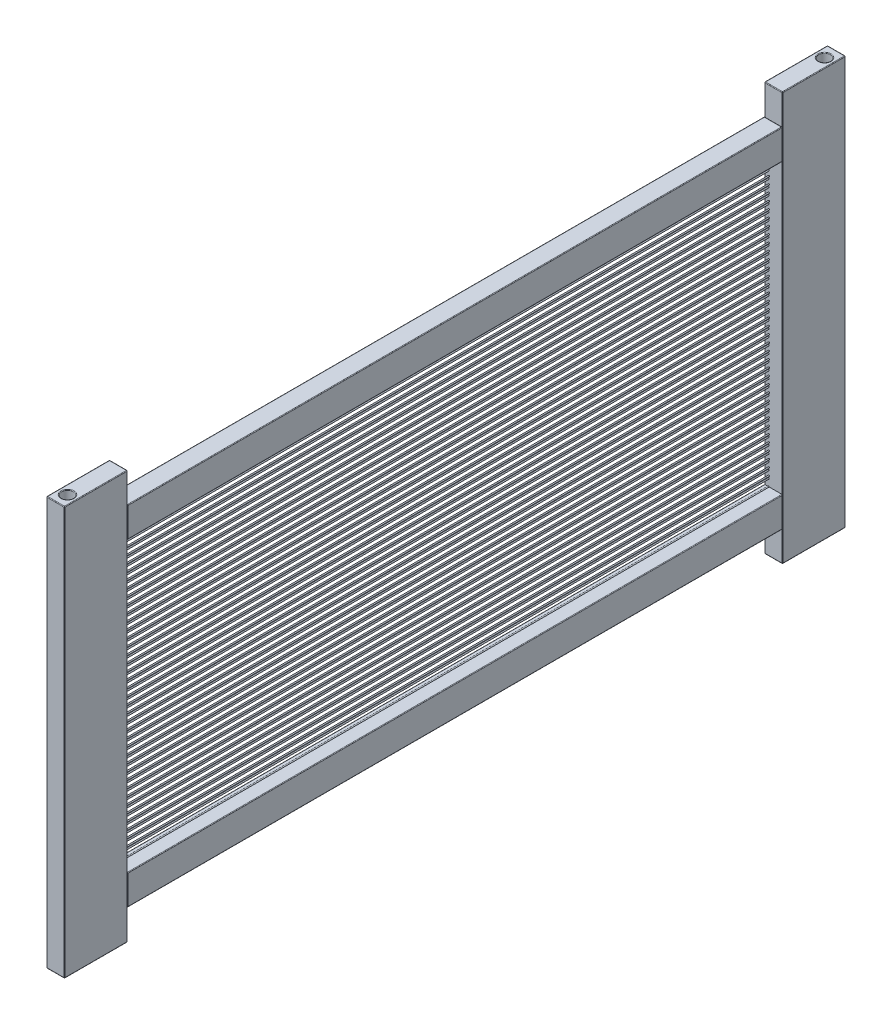
from build123d import *

# Parameters (mm, degrees)
SKETCH_1_W          = 30
SKETCH_1_H          = 105
EXTRUDE_1_DEPTH     = 680
EXTRUDE_1_2_DEPTH   = 680
SKETCH_2_R          = 10
CUT_EXTRUDE_1_DEPTH = 1421.873410969
SKETCH_6_W          = 30
SKETCH_6_H          = 50
EXTRUDE_2_DEPTH     = 1090
EXTRUDE_2_2_DEPTH   = 1090
SKETCH_7_R          = 1
EXTRUDE_3_DEPTH     = 1090
FILLET_1_R          = 1
FILLET_2_R          = 1
FILLET_3_R          = 1
FILLET_4_R          = 1


with BuildPart() as part:
    # 草图1 → 凸台-拉伸1 (new body)
    with BuildSketch(Plane(origin=(0, 0, 0), x_dir=(1, 0, 0), z_dir=(0, 1, 0))):
        Rectangle(SKETCH_1_W, SKETCH_1_H)
    extrude(amount=EXTRUDE_1_DEPTH)


with BuildPart() as body_2:
    # 草图1 → Extrude 1 2 (new body)
    with BuildSketch(Plane(origin=(0, 0, 0), x_dir=(1, 0, 0), z_dir=(0, 1, 0))):
        with Locations((0, 1195)):
            Rectangle(SKETCH_1_W, SKETCH_1_H)
    extrude(amount=EXTRUDE_1_2_DEPTH)


with BuildPart() as cut_extrude_1_tool:
    # 草图2 → 切除-拉伸1 (new, through all)
    with BuildSketch(Plane.XZ):
        with Locations(Location((0, 32.5, 0), (0, 0, 270))):
            Circle(SKETCH_2_R)
        with Locations(Location((0, -1227.5, 0), (0, 0, 270))):
            Circle(SKETCH_2_R)
    extrude(amount=-CUT_EXTRUDE_1_DEPTH)


with BuildPart() as part_1:
    add(part.part)

    # 切除-拉伸1: cut by cut_extrude_1_tool
    add(cut_extrude_1_tool.part, mode=Mode.SUBTRACT)

    # 圆角1
    fillet_1_edges = [part_1.edges().sort_by_distance(p)[0] for p in [
        (-15, 680, 0),
        (0, 680, 52.5),
        (0, 680, 42.5),
        (0, 0, 42.5),
        (15, 680, 0),
        (0, 0, 52.5),
        (-15, 0, 0),
        (0, 0, -52.5),
        (15, 0, 0),
        (0, 680, -52.5),
        (15, 340, 52.5),
        (-15, 340, 52.5),
        (-15, 340, -52.5),
        (15, 340, -52.5),
    ]]
    fillet(fillet_1_edges, radius=FILLET_1_R)


with BuildPart() as body_2_1:
    add(body_2.part)

    # 切除-拉伸1: cut by cut_extrude_1_tool
    add(cut_extrude_1_tool.part, mode=Mode.SUBTRACT)

    # 圆角3
    fillet_3_edges = [body_2_1.edges().sort_by_distance(p)[0] for p in [
        (-15, 680, -1195),
        (0, 680, -1142.5),
        (0, 680, -1217.5),
        (15, 680, -1195),
        (0, 0, -1142.5),
        (-15, 0, -1195),
        (0, 0, -1247.5),
        (15, 0, -1195),
        (0, 680, -1247.5),
        (15, 340, -1142.5),
        (-15, 340, -1142.5),
        (-15, 340, -1247.5),
        (15, 340, -1247.5),
    ]]
    fillet(fillet_3_edges, radius=FILLET_3_R)


with BuildPart() as body_3:
    # 草图6 → 凸台-拉伸2 (new body)
    with BuildSketch(Plane.XY.offset(-1142.5)):
        with Locations((0, 75)):
            Rectangle(SKETCH_6_W, SKETCH_6_H)
    extrude(amount=EXTRUDE_2_DEPTH)

    # 圆角4
    fillet_4_edges = [body_3.edges().sort_by_distance(p)[0] for p in [
        (0, 50, -1142.5),
        (15, 50, -597.5),
        (15, 75, -1142.5),
        (15, 100, -597.5),
        (-15, 75, -52.5),
        (0, 50, -52.5),
        (15, 75, -52.5),
        (-15, 100, -597.5),
        (-15, 75, -1142.5),
        (-15, 50, -597.5),
    ]]
    fillet(fillet_4_edges, radius=FILLET_4_R)


with BuildPart() as body_4:
    # 草图6 → Extrude 2 2 (new body)
    with BuildSketch(Plane.XY.offset(-1142.5)):
        with Locations((0, 605)):
            Rectangle(SKETCH_6_W, SKETCH_6_H)
    extrude(amount=EXTRUDE_2_2_DEPTH)

    # 圆角2
    fillet_2_edges = [body_4.edges().sort_by_distance(p)[0] for p in [
        (15, 580, -597.5),
        (15, 605, -1142.5),
        (15, 630, -597.5),
        (0, 630, -1142.5),
        (0, 630, -52.5),
        (-15, 605, -52.5),
        (15, 605, -52.5),
        (-15, 630, -597.5),
        (-15, 605, -1142.5),
        (-15, 580, -597.5),
    ]]
    fillet(fillet_2_edges, radius=FILLET_2_R)


with BuildPart() as body_5:
    # 草图7 → 凸台-拉伸3 (new body)
    with BuildSketch(Plane.XY.offset(-1142.5)):
        with Locations((-8, 568)):
            Circle(SKETCH_7_R)
        with Locations((-7.551054028, 583.993700245)):
            Circle(SKETCH_7_R)
        with Locations((-8, 556)):
            Circle(SKETCH_7_R)
        with Locations((-7.551054028, 571.993700245)):
            Circle(SKETCH_7_R)
        with Locations((-8, 544)):
            Circle(SKETCH_7_R)
        with Locations((-7.551054028, 559.993700245)):
            Circle(SKETCH_7_R)
        with Locations((-8, 532)):
            Circle(SKETCH_7_R)
        with Locations((-7.551054028, 547.993700245)):
            Circle(SKETCH_7_R)
        with Locations((-8, 520)):
            Circle(SKETCH_7_R)
        with Locations((-7.551054028, 535.993700245)):
            Circle(SKETCH_7_R)
        with Locations((-8, 508)):
            Circle(SKETCH_7_R)
        with Locations((-7.551054028, 523.993700245)):
            Circle(SKETCH_7_R)
        with Locations((-8, 496)):
            Circle(SKETCH_7_R)
        with Locations((-7.551054028, 511.993700245)):
            Circle(SKETCH_7_R)
        with Locations((-8, 484)):
            Circle(SKETCH_7_R)
        with Locations((-7.551054028, 499.993700245)):
            Circle(SKETCH_7_R)
        with Locations((-8, 472)):
            Circle(SKETCH_7_R)
        with Locations((-7.551054028, 487.993700245)):
            Circle(SKETCH_7_R)
        with Locations((-8, 460)):
            Circle(SKETCH_7_R)
        with Locations((-7.551054028, 475.993700245)):
            Circle(SKETCH_7_R)
        with Locations((-8, 448)):
            Circle(SKETCH_7_R)
        with Locations((-7.551054028, 463.993700245)):
            Circle(SKETCH_7_R)
        with Locations((-8, 436)):
            Circle(SKETCH_7_R)
        with Locations((-7.551054028, 451.993700245)):
            Circle(SKETCH_7_R)
        with Locations((-8, 424)):
            Circle(SKETCH_7_R)
        with Locations((-7.551054028, 439.993700245)):
            Circle(SKETCH_7_R)
        with Locations((-8, 412)):
            Circle(SKETCH_7_R)
        with Locations((-7.551054028, 427.993700245)):
            Circle(SKETCH_7_R)
        with Locations((-8, 400)):
            Circle(SKETCH_7_R)
        with Locations((-7.551054028, 415.993700245)):
            Circle(SKETCH_7_R)
        with Locations((-8, 388)):
            Circle(SKETCH_7_R)
        with Locations((-7.551054028, 403.993700245)):
            Circle(SKETCH_7_R)
        with Locations((-8, 376)):
            Circle(SKETCH_7_R)
        with Locations((-7.551054028, 391.993700245)):
            Circle(SKETCH_7_R)
        with Locations((-8, 364)):
            Circle(SKETCH_7_R)
        with Locations((-7.551054028, 379.993700245)):
            Circle(SKETCH_7_R)
        with Locations((-8, 352)):
            Circle(SKETCH_7_R)
        with Locations((-7.551054028, 367.993700245)):
            Circle(SKETCH_7_R)
        with Locations((-8, 340)):
            Circle(SKETCH_7_R)
        with Locations((-7.551054028, 355.993700245)):
            Circle(SKETCH_7_R)
        with Locations((-8, 328)):
            Circle(SKETCH_7_R)
        with Locations((-7.551054028, 343.993700245)):
            Circle(SKETCH_7_R)
        with Locations((-8, 316)):
            Circle(SKETCH_7_R)
        with Locations((-7.551054028, 331.993700245)):
            Circle(SKETCH_7_R)
        with Locations((-8, 304)):
            Circle(SKETCH_7_R)
        with Locations((-7.551054028, 319.993700245)):
            Circle(SKETCH_7_R)
        with Locations((-8, 292)):
            Circle(SKETCH_7_R)
        with Locations((-7.551054028, 307.993700245)):
            Circle(SKETCH_7_R)
        with Locations((-8, 280)):
            Circle(SKETCH_7_R)
        with Locations((-7.551054028, 295.993700245)):
            Circle(SKETCH_7_R)
        with Locations((-8, 268)):
            Circle(SKETCH_7_R)
        with Locations((-7.551054028, 283.993700245)):
            Circle(SKETCH_7_R)
        with Locations((-8, 256)):
            Circle(SKETCH_7_R)
        with Locations((-7.551054028, 271.993700245)):
            Circle(SKETCH_7_R)
        with Locations((-8, 244)):
            Circle(SKETCH_7_R)
        with Locations((-7.551054028, 259.993700245)):
            Circle(SKETCH_7_R)
        with Locations((-8, 232)):
            Circle(SKETCH_7_R)
        with Locations((-7.551054028, 247.993700245)):
            Circle(SKETCH_7_R)
        with Locations((-8, 220)):
            Circle(SKETCH_7_R)
        with Locations((-7.551054028, 235.993700245)):
            Circle(SKETCH_7_R)
        with Locations((-8, 208)):
            Circle(SKETCH_7_R)
        with Locations((-7.551054028, 223.993700245)):
            Circle(SKETCH_7_R)
        with Locations((-8, 196)):
            Circle(SKETCH_7_R)
        with Locations((-7.551054028, 211.993700245)):
            Circle(SKETCH_7_R)
        with Locations((-8, 184)):
            Circle(SKETCH_7_R)
        with Locations((-7.551054028, 199.993700245)):
            Circle(SKETCH_7_R)
        with Locations((-8, 172)):
            Circle(SKETCH_7_R)
        with Locations((-7.551054028, 187.993700245)):
            Circle(SKETCH_7_R)
        with Locations((-8, 160)):
            Circle(SKETCH_7_R)
        with Locations((-7.551054028, 175.993700245)):
            Circle(SKETCH_7_R)
        with Locations((-8, 148)):
            Circle(SKETCH_7_R)
        with Locations((-7.551054028, 163.993700245)):
            Circle(SKETCH_7_R)
        with Locations((-8, 136)):
            Circle(SKETCH_7_R)
        with Locations((-7.551054028, 151.993700245)):
            Circle(SKETCH_7_R)
        with Locations((-8, 124)):
            Circle(SKETCH_7_R)
        with Locations((-7.551054028, 139.993700245)):
            Circle(SKETCH_7_R)
        with Locations((-8, 112)):
            Circle(SKETCH_7_R)
        with Locations((-7.551054028, 127.993700245)):
            Circle(SKETCH_7_R)
        with Locations((-8, 100)):
            Circle(SKETCH_7_R)
        with Locations((-7.551054028, 115.993700245)):
            Circle(SKETCH_7_R)
    extrude(amount=EXTRUDE_3_DEPTH)


solid = Compound([part_1.part, body_2_1.part, body_3.part, body_4.part, body_5.part])
